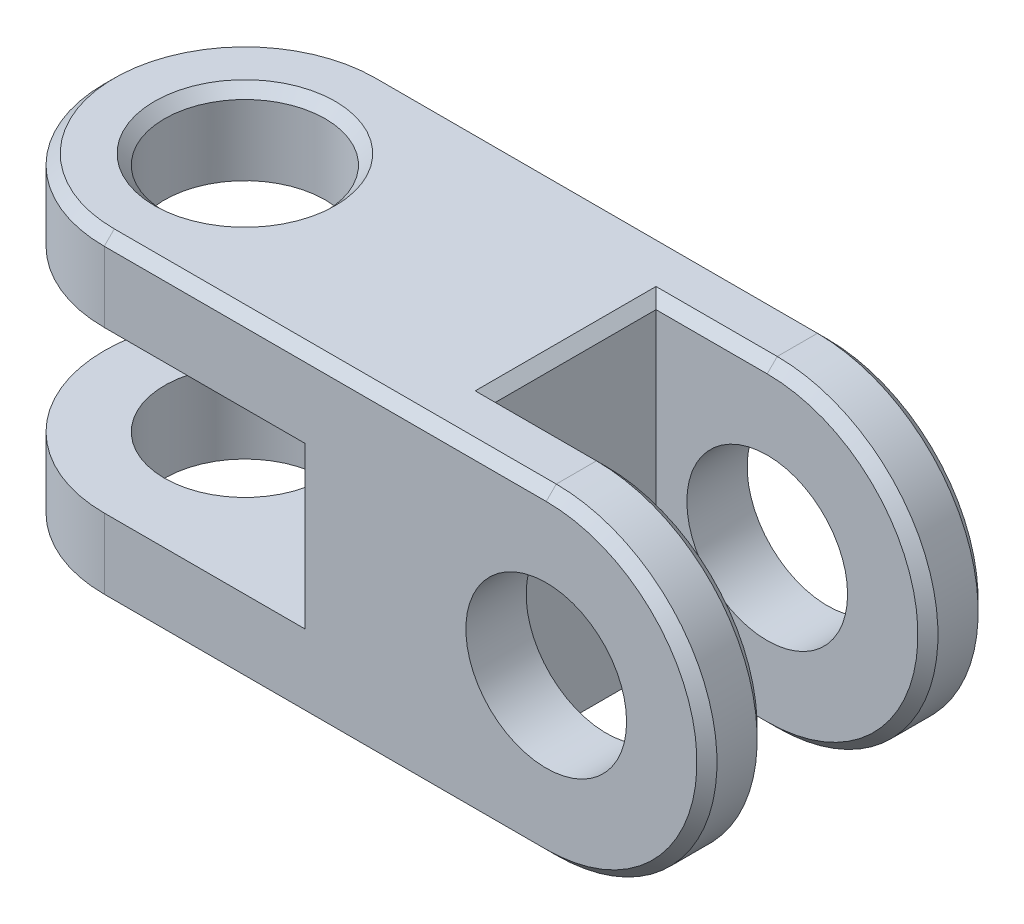
SolidWorks part; units mm, degrees
material "1060 Alloy"
ref_plane "Front Plane" through (0, 0, 0) normal (0, 0, 1) x (1, 0, 0)
ref_plane "Top Plane" through (0, 0, 0) normal (0, 1, 0) x (1, 0, 0)
ref_plane "Right Plane" through (0, 0, 0) normal (1, 0, 0) x (0, 0, -1)
sketch "Sketch1" plane through (0, 0, 0) normal (0, 1, 0) x (1, 0, 0)
  line L1 (0, 7) -> (30, 7)
  line L3 (0, -7) -> (30, -7)
  line L4 (30, 7) -> (30, -7)
  circle A0 centre (0, 0) radius 4
  arc A1 (0, 7) -> (0, -7) centre (0, 0) ccw
  dimension "D1" = 8
  dimension "D2" = 14
  dimension "D3" = 14
extrude "Boss-Extrude1" add sketch "Sketch1" along normal blind 16
sketch "Sketch2" plane through (0, 16, 0) normal (0, 1, 0) x (1, 0, 0)
  line L0 (30, -7) -> (30, 7) construction
  line L1 (30, 4) -> (16.4648, 4)
  line L2 (30, 4) -> (30, -4)
  line L3 (30, -4) -> (16.4648, -4)
  line L4 (16.4648, 4) -> (16.4648, -4)
  line L5 (30, 7) -> (0, 7) construction
  line L6 (0, -7) -> (30, -7) construction
  dimension "D1" = 3
  dimension "D2" = 3
extrude "Cut-Extrude1" cut sketch "Sketch2" against normal blind 16
sketch "Sketch3" plane through (0, 0, 7) normal (0, 0, 1) x (1, 0, 0)
  line L0 (30, 16) -> (30, 0) construction
  line L1 (22, 16) -> (30, 16)
  line L2 (30, 16) -> (30, 0)
  line L3 (30, 0) -> (22, 0)
  arc A0 (22, 0) -> (22, 16) centre (22, 8) ccw
  circle A1 centre (22, 8) radius 4
  line M3 (0, 0) -> (30, 0)
  line M4 (30, 0) -> (30, 16)
  line M5 (30, 16) -> (0, 16)
  dimension "D1" = 16
  dimension "D2" = 8
  dimension "D3" = 8
extrude "Cut-Extrude2" cut sketch "Sketch3" against normal blind 16 contours A0 L2 M5 | A0 M3 M4 | A1
sketch "Sketch4" plane through (0, 0, 0) normal (1, 0, 0) x (0, 0, -1)
  line L0 (-7, 16) -> (-7, 0) construction
  line L1 (-7, 12) -> (7, 12)
  line L2 (-7, 12) -> (-7, 4)
  line L3 (-7, 4) -> (7, 4)
  line L4 (7, 12) -> (7, 4)
  line L5 (7, 0) -> (7, 16) construction
  line L6 (4, 0) -> (-4, 0) construction
  dimension "D1" = 8
  dimension "D2" = 4
extrude "Cut-Extrude3" cut sketch "Sketch4" against normal blind 16 and the other way blind 10
chamfer "Chamfer1" distance 0.5 angle 45 16 edges at (0, 16, 4) (19.2324, 0, -4) (19.2324, 0, 4) (30, 8, -4) (30, 8, 4) (19.2324, 16, -4) (16.4648, 16, 0) (19.2324, 16, 4) (-7, 0, 0) (11, 0, 7) (11, 0, -7) (30, 8, 7) (30, 8, -7) (11, 16, 7) (-7, 16, 0) (11, 16, -7)
scale "Scale1" scale about origin uniform scaling yes scale factor 0.5
